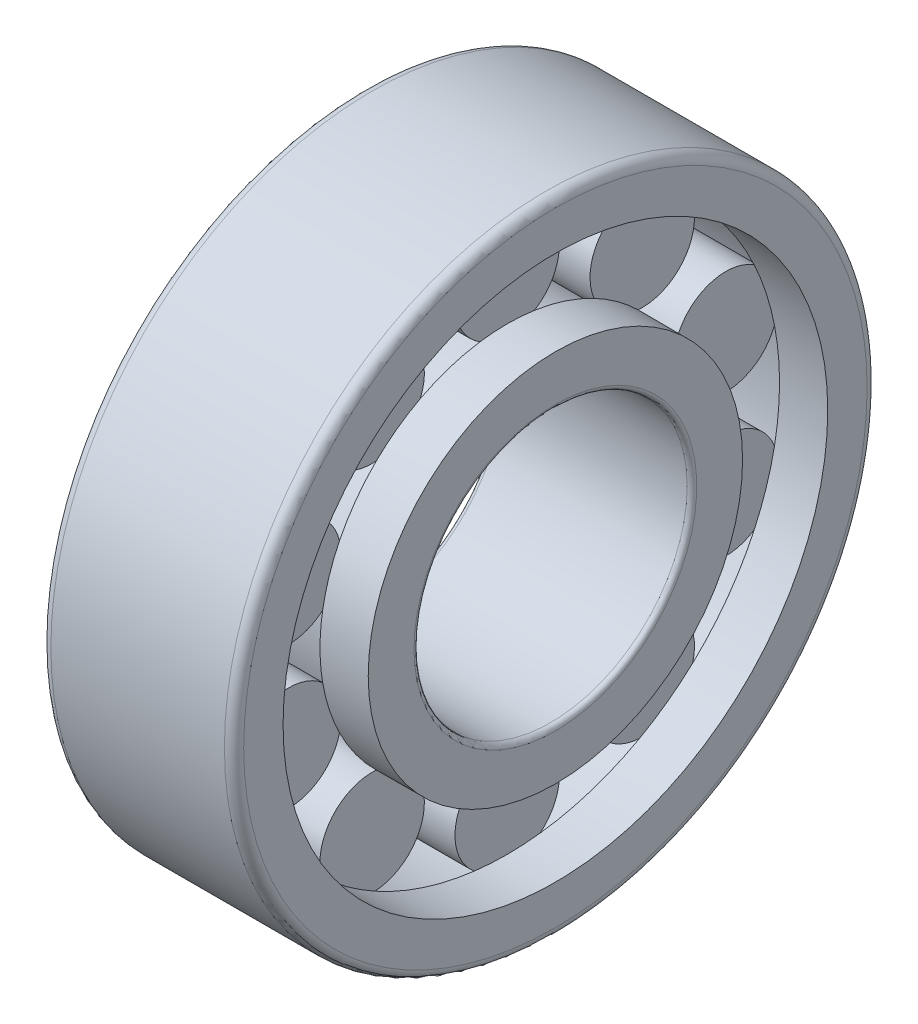
from build123d import *

# Parameters (mm, degrees)
SKETCH_3_W               = 6
SKETCH_3_H               = 3.2501
PATTERN_CIRCULAR_1_COUNT = 10


with BuildPart() as part:
    # 草图2 → Revolve 705 (revolve)
    with BuildSketch(Plane.XY, mode=Mode.PRIVATE) as revolve_705_sk:
        with BuildLine():
            Line((3, 11.05), (9, 11.05))
            Line((9, 11.05), (9, 11.65))
            Line((9, 11.65), (12, 11.65))
            Line((12, 11.65), (12, 8.8))
            ThreePointArc((12, 8.8), (11.912132034, 8.587867966), (11.7, 8.5))
            Line((11.7, 8.5), (0.3, 8.5))
            ThreePointArc((0.3, 8.5), (0.087867966, 8.587867966), (0, 8.8))
            Line((0, 8.8), (0, 11.65))
            Line((0, 11.65), (3, 11.65))
            Line((3, 11.65), (3, 11.05))
        make_face()
    revolve(revolve_705_sk.sketch.rotate(Axis((-10.080094127, 0, 0), (1, 0, 0)), 90), axis=Axis((-10.080094127, 0, 0), (1, 0, 0)))

    # 草图3 → 凸台-旋转1 (revolve)
    with BuildSketch(Plane.XY):
        with Locations((6, 12.67495)):
            Rectangle(SKETCH_3_W, SKETCH_3_H)
    revolve_1 = revolve(axis=Axis((-1.603948851, 14.3, 0), (1, 0, 0)))

    # 草图4 → 凸台-旋转2 (revolve)
    with BuildSketch(Plane.XY, mode=Mode.PRIVATE) as revolve_2_sk:
        with BuildLine():
            Line((9, 16.95), (12, 16.95))
            Line((12, 16.95), (12, 19.4))
            ThreePointArc((12, 19.4), (11.824264069, 19.824264069), (11.4, 20))
            Line((11.4, 20), (0.6, 20))
            ThreePointArc((0.6, 20), (0.175735931, 19.824264069), (0, 19.4))
            Line((0, 19.4), (0, 16.95))
            Line((0, 16.95), (3, 16.95))
            Line((3, 16.95), (3, 17.55))
            Line((3, 17.55), (9, 17.55))
            Line((9, 17.55), (9, 16.95))
        make_face()
    revolve(revolve_2_sk.sketch.rotate(Axis((0, 0, 0), (1, 0, 0)), 90), axis=Axis((0, 0, 0), (1, 0, 0)))

    # 阵列(圆周)1: 凸台-旋转1 ×10 about axis
    pattern_circular_1_axis = Axis((0, 0, 0), (1, 0, 0))
    for i in range(1, PATTERN_CIRCULAR_1_COUNT):
        add(revolve_1.rotate(pattern_circular_1_axis, i * 360 / PATTERN_CIRCULAR_1_COUNT))


solid = part.part
